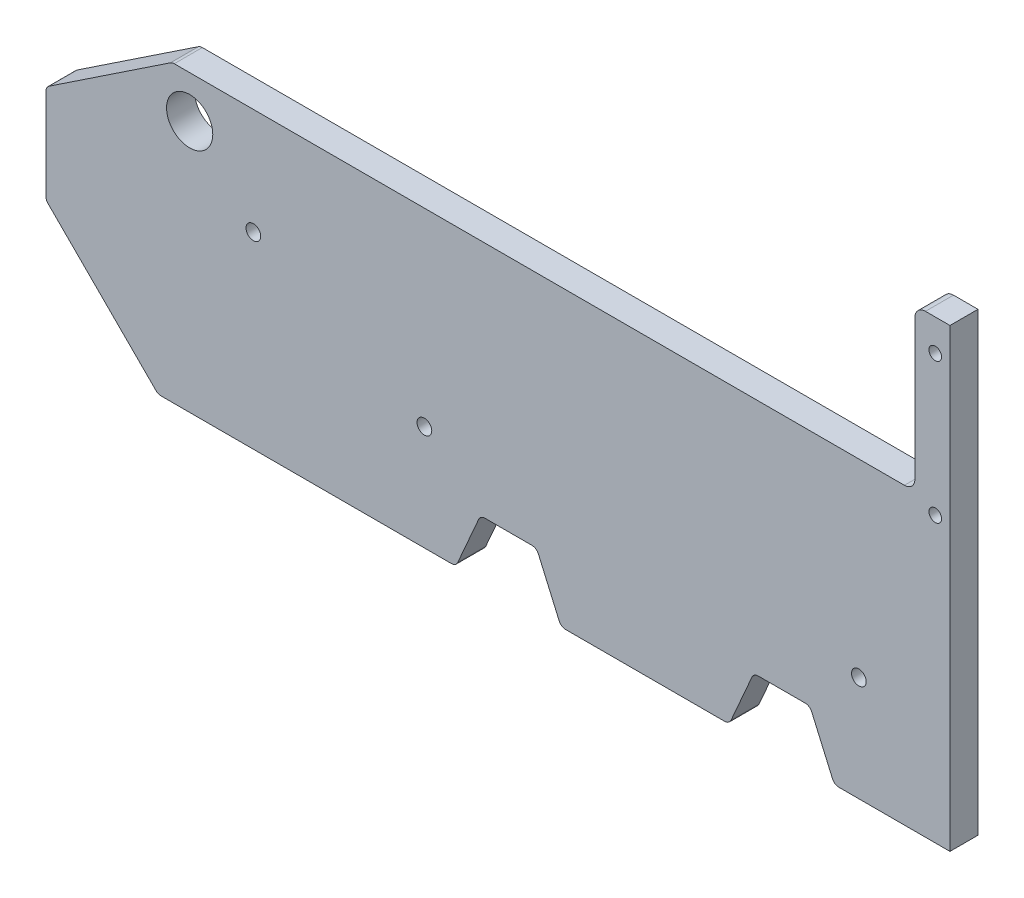
from build123d import *

# Parameters (mm, degrees)
SKETCH1_R           = 33
SKETCH1_R_2         = 9
BOSS_EXTRUDE1_DEPTH = 40
CHAMFER2_SIZE       = 180
CHAMFER2_SIZE2      = 120
CHAMFER3_SIZE       = 160
M24_TAPPED_HOLE1_D  = 21
FILLET1_R           = 15
CUT_EXTRUDE1_DEPTH  = 1446.060552365
FILLET2_R           = 10
FILLET3_R           = 10


with BuildPart() as part:
    # Sketch1 → Boss-Extrude1 (new body)
    with BuildSketch(Plane.XY):
        Polygon((1240, 420), (1240, 650), (1290, 650), (1290, 0), (0, 0), (0, 420), align=None)
        with Locations((205, 360)):
            Circle(SKETCH1_R, mode=Mode.SUBTRACT)
        with Locations((1269, 405)):
            Circle(SKETCH1_R_2, mode=Mode.SUBTRACT)
        with Locations((1269, 605)):
            Circle(SKETCH1_R_2, mode=Mode.SUBTRACT)
    extrude(amount=BOSS_EXTRUDE1_DEPTH)

    # Chamfer2
    chamfer2_edges = [part.edges().sort_by_distance(p)[0] for p in [
        (0, 420, 20),
    ]]
    chamfer2_side = [part.faces().sort_by_distance(p)[0] for p in [
        (620, 420, 20),
    ]]
    chamfer(chamfer2_edges, length=CHAMFER2_SIZE, length2=CHAMFER2_SIZE2, reference=chamfer2_side[0])

    # Chamfer3
    chamfer3_edges = [part.edges().sort_by_distance(p)[0] for p in [
        (0, 0, 20),
    ]]
    chamfer(chamfer3_edges, length=CHAMFER3_SIZE)

    # M24 Tapped Hole1 (through all)
    with Locations(Plane(origin=(540, 150, 40), x_dir=(1, 0, 0), z_dir=(0, 0, 1))):
        with Locations((0, 0), (620, 0), (-244.064633972, 118.316259911)):
            Hole(M24_TAPPED_HOLE1_D / 2)

    # Fillet1
    fillet1_edges = [part.edges().sort_by_distance(p)[0] for p in [
        (1240, 420, 20),
        (1240, 650, 20),
    ]]
    fillet(fillet1_edges, radius=FILLET1_R)

    # Sketch2 → Cut-Extrude1 (cut, through all)
    with BuildSketch(Plane.XY.offset(40)):
        Polygon((585, 0), (735, 0), (700, 80), (620, 80), align=None)
        Polygon((975, 0), (1125, 0), (1090, 80), (1010, 80), align=None)
    extrude(amount=-CUT_EXTRUDE1_DEPTH, mode=Mode.SUBTRACT)

    # Fillet2
    fillet2_edges = [part.edges().sort_by_distance(p)[0] for p in [
        (700, 80, 20),
        (735, 0, 20),
        (585, 0, 20),
        (620, 80, 20),
        (1010, 80, 20),
        (1090, 80, 20),
        (1125, 0, 20),
        (975, 0, 20),
    ]]
    fillet(fillet2_edges, radius=FILLET2_R)

    # Fillet3
    fillet3_edges = [part.edges().sort_by_distance(p)[0] for p in [
        (0, 300, 20),
        (180, 420, 20),
        (160, 0, 20),
        (0, 160, 20),
    ]]
    fillet(fillet3_edges, radius=FILLET3_R)


solid = part.part
